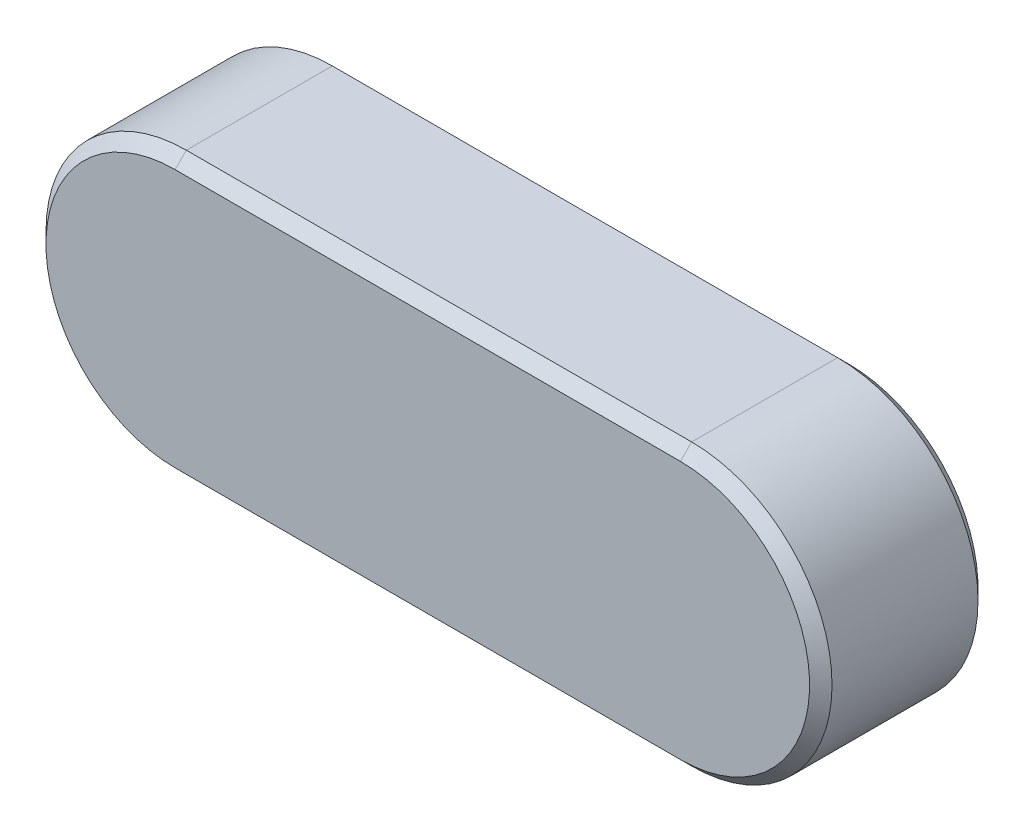
from build123d import *

# Parameters (mm, degrees)
BASEKEY_DEPTH = 6
CHAMFER1_SIZE = 0.8


with BuildPart() as part:
    # Sketch1 → BaseKey (new, symmetric)
    with BuildSketch(Plane.XY):
        with BuildLine():
            Line((-36, 10), (0, 10))
            ThreePointArc((0, 10), (10, 0), (0, -10))
            Line((0, -10), (-36, -10))
            ThreePointArc((-36, -10), (-46, 0), (-36, 10))
        make_face()
    extrude(amount=BASEKEY_DEPTH, both=True)

    # Chamfer1
    chamfer1_edges = [part.edges().sort_by_distance(p)[0] for p in [
        (10, 0, 6),
        (-18, 10, 6),
        (-46, 0, 6),
        (-18, 10, -6),
        (10, 0, -6),
        (-18, -10, -6),
        (-46, 0, -6),
        (-18, -10, 6),
    ]]
    chamfer(chamfer1_edges, length=CHAMFER1_SIZE)


solid = part.part
